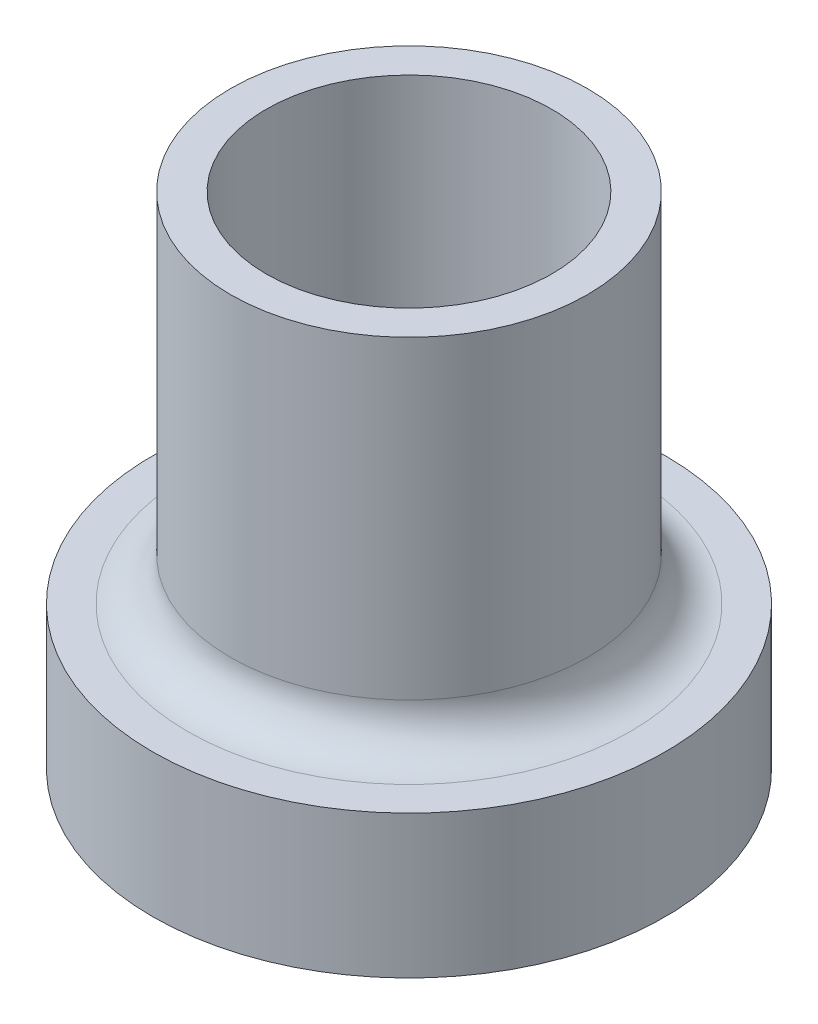
from build123d import *


with BuildPart() as part:
    # Sketch1 → Revolve2 (revolve)
    with BuildSketch(Plane.XY, mode=Mode.PRIVATE) as revolve2_sk:
        with BuildLine():
            Line((-10, 28.836781592), (-12.5, 28.836781592))
            Line((-12.5, 28.836781592), (-12.5, 6.836781592))
            ThreePointArc((-12.5, 6.836781592), (-13.378679656, 4.715461249), (-15.5, 3.836781592))
            Line((-15.5, 3.836781592), (-17.956309532, 3.836781592))
            Line((-17.956309532, 3.836781592), (-17.956309532, -6.163218408))
            Line((-17.956309532, -6.163218408), (-15.5, -6.163218408))
            ThreePointArc((-15.5, -6.163218408), (-11.507640786, -3.017340367), (-10, 1.836781592))
            Line((-10, 1.836781592), (-10, 28.836781592))
        make_face()
    revolve(revolve2_sk.sketch.rotate(Axis((0, 10.886363636, 0), (0, -1, 0)), 270), axis=Axis((0, 10.886363636, 0), (0, -1, 0)))


solid = part.part
